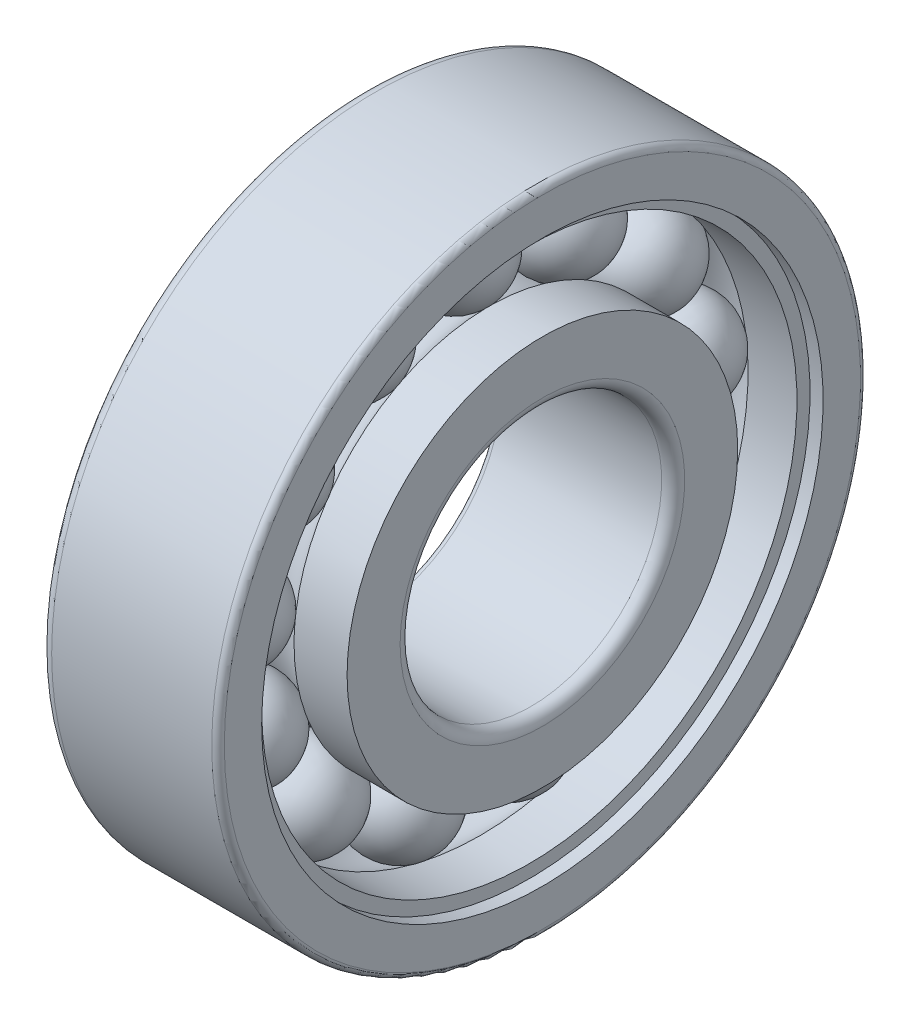
from build123d import *

# Parameters (mm, degrees)
CIRCULAR_PATTERN1_COUNT = 13
FILLET1_R               = 1.1
FILLET2_R               = 0.6


with BuildPart() as part:
    # Sketch1 → Revolve1 (revolve)
    with BuildSketch(Plane.XY):
        with BuildLine():
            Line((-4.625, 21.75), (4.625, 21.75))
            ThreePointArc((4.625, 21.75), (0, 17.125), (-4.625, 21.75))
        make_face()
    revolve1 = revolve(axis=Axis((-3.091912561, 21.75, 0), (1, 0, 0)))

    # Sketch2 → Revolve2 (revolve)
    with BuildSketch(Plane.XY, mode=Mode.PRIVATE) as revolve2_sk:
        with BuildLine():
            Line((-8.5, 18.666666667), (-3.433843409, 18.666666667))
            ThreePointArc((-3.433843409, 18.666666667), (0, 17.135), (3.433843409, 18.666666667))
            Line((3.433843409, 18.666666667), (8.5, 18.666666667))
            Line((8.5, 18.666666667), (8.5, 12.5))
            Line((8.5, 12.5), (-8.5, 12.5))
            Line((-8.5, 12.5), (-8.5, 18.666666667))
        make_face()
    revolve(revolve2_sk.sketch.rotate(Axis((-2.992358943, 0, 0), (1, 0, 0)), 90), axis=Axis((-2.992358943, 0, 0), (1, 0, 0)))

    # Sketch3 → Revolve3 (revolve)
    with BuildSketch(Plane.XY, mode=Mode.PRIVATE) as revolve3_sk:
        with BuildLine():
            Line((-8.5, 24.833333333), (-8.5, 31))
            Line((-8.5, 31), (8.5, 31))
            Line((8.5, 31), (8.5, 26.828333333))
            Line((8.5, 26.828333333), (7.25, 26.828333333))
            Line((7.25, 26.828333333), (7.25, 25.578333333))
            Line((7.25, 25.578333333), (2.577225037, 25.578333333))
            ThreePointArc((2.577225037, 25.578333333), (-0.56763105, 26.329958514), (-3.433843409, 24.833333333))
            Line((-3.433843409, 24.833333333), (-8.5, 24.833333333))
        make_face()
    revolve(revolve3_sk.sketch.rotate(Axis((-2.992358943, 0, 0), (1, 0, 0)), 90), axis=Axis((-2.992358943, 0, 0), (1, 0, 0)))

    # Circular-Pattern1: Revolve1 ×13 about axis
    circular_pattern1_axis = Axis((0, 0, 0), (1, 0, 0))
    for i in range(1, CIRCULAR_PATTERN1_COUNT):
        add(revolve1.rotate(circular_pattern1_axis, i * 360 / CIRCULAR_PATTERN1_COUNT))

    # Fillet1
    fillet1_edges = [part.edges().sort_by_distance(p)[0] for p in [
        (-8.5, 0, -31),
        (8.5, 0, -12.5),
    ]]
    fillet(fillet1_edges, radius=FILLET1_R)

    # Fillet2
    fillet2_edges = [part.edges().sort_by_distance(p)[0] for p in [
        (8.5, 0, -31),
        (-8.5, 0, -12.5),
    ]]
    fillet(fillet2_edges, radius=FILLET2_R)


solid = part.part
